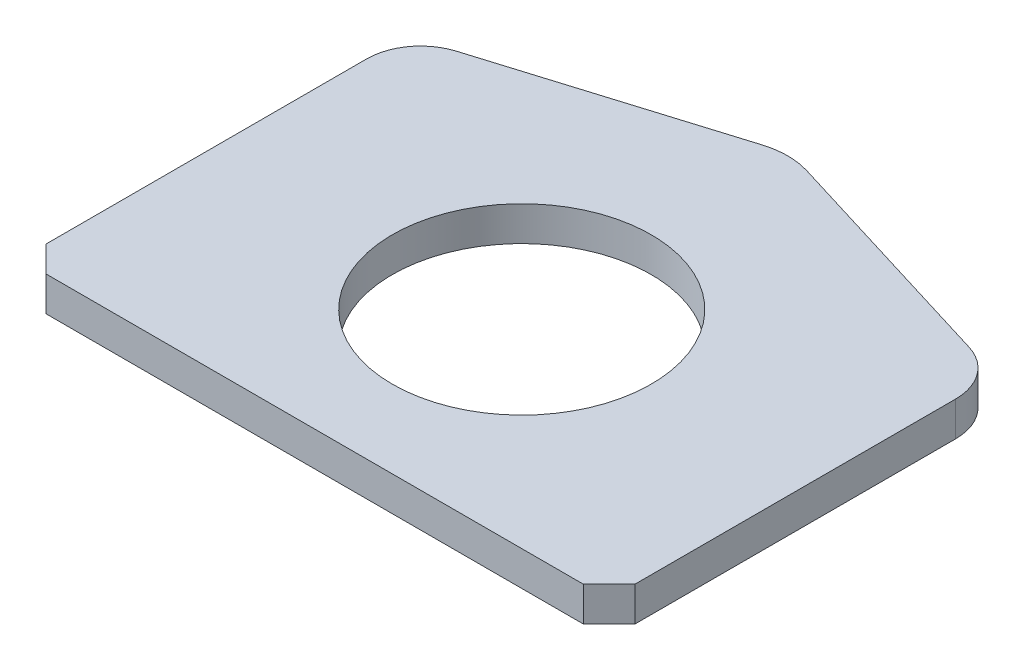
SolidWorks part; units mm, degrees
ref_plane "Front Plane" through (0, 0, 0) normal (0, 0, 1) x (1, 0, 0)
ref_plane "Top Plane" through (0, 0, 0) normal (0, 1, 0) x (1, 0, 0)
ref_plane "Right Plane" through (0, 0, 0) normal (1, 0, 0) x (0, 0, -1)
sketch "Sketch1" plane through (0, 0, 0) normal (0, 1, 0) x (1, 0, 0)
  line L0 (-124.5, 0) -> (124.5, 0)
  line L1 (136.5, 12) -> (136.5, 160.6)
  line L2 (10.2522, 217.7648) -> (118.823, 184.5034)
  line L3 (0, 0) -> (0, 257.778) construction
  line L4 (124.5, 0) -> (136.5, 12)
  line L5 (-124.5, 0) -> (-136.5, 12)
  line L6 (-136.5, 12) -> (-136.5, 160.6)
  line L7 (-10.2522, 217.7648) -> (-118.823, 184.5034)
  arc A0 (136.5, 160.6) -> (118.823, 184.5034) centre (111.5, 160.6) ccw
  arc A1 (10.2522, 217.7648) -> (-10.2522, 217.7648) centre (0, 184.3) ccw
  arc A2 (-136.5, 160.6) -> (-118.823, 184.5034) centre (-111.5, 160.6) cw
  circle A3 centre (0, 96) radius 60
  point P7 (136.5, 0)
  point P16 (-136.5, 0)
  dimension "D2" = 70
  dimension "D5" = 50
  dimension "D6" = 120
  dimension "D1" = 273
  dimension "D3" = 184.3
  dimension "D4" = 160.6
  dimension "D7" = 96
extrude "Boss-Extrude1" add sketch "Sketch1" along normal blind 16
